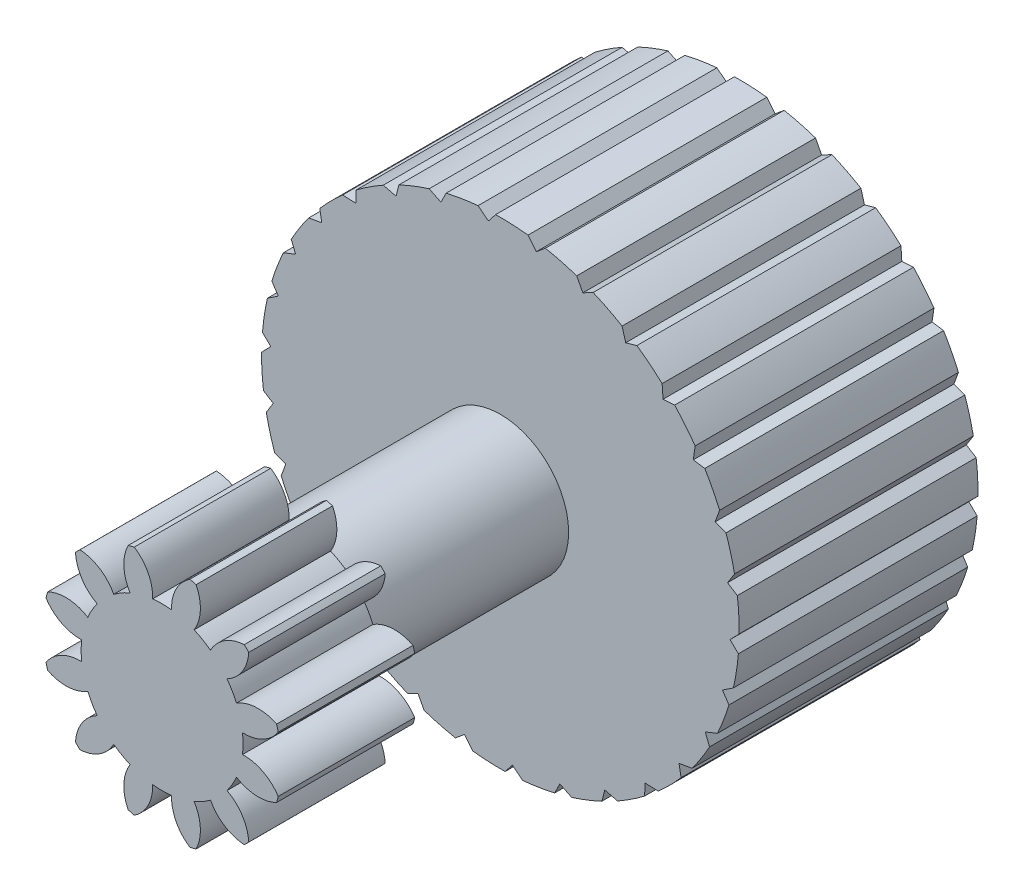
SolidWorks part; units mm, degrees
ref_plane "Front Plane" through (0, 0, 0) normal (0, 0, 1) x (1, 0, 0)
ref_plane "Top Plane" through (0, 0, 0) normal (0, 1, 0) x (1, 0, 0)
ref_plane "Right Plane" through (0, 0, 0) normal (1, 0, 0) x (0, 0, -1)
other "Configuration Table"
sketch "Sketch1" plane through (0, 0, 0) normal (0, 0, 1) x (1, 0, 0)
  circle A0 centre (0, 0) radius 1
  dimension "D1" = 2
extrude "Boss-Extrude1" add sketch "Sketch1" along normal blind 3
sketch "Sketch2" plane through (0, 0, 3) normal (0, 0, 1) x (1, 0, 0)
  arc A0 (-1.2279, 1.1338) -> (-0.9093, 0.6388) centre (-0.629, 1.1693) ccw
  arc A1 (-0.9093, 0.6388) -> (-1.0478, 0.3989) centre (0.0419, -0.0703) ccw
  arc A2 (-1.0478, 0.3989) -> (-1.6358, 0.4273) centre (-1.3671, -0.1091) ccw
  arc A3 (-1.6358, 0.4273) -> (-1.6599, 0.3375) centre (0.0419, -0.0703) ccw
  arc A4 (-1.6599, 0.3375) -> (-1.1365, 0.0682) centre (-1.1589, 0.6677) ccw
  arc A5 (-1.1365, 0.0682) -> (-1.1365, -0.2088) centre (0.0419, -0.0703) ccw
  arc A6 (-1.1365, -0.2088) -> (-1.6599, -0.4782) centre (-1.1589, -0.8084) ccw
  arc A7 (-1.6599, -0.4782) -> (-1.6358, -0.568) centre (0.0419, -0.0703) ccw
  arc A8 (-1.6358, -0.568) -> (-1.0478, -0.5396) centre (-1.3671, -0.0316) ccw
  arc A9 (-1.0478, -0.5396) -> (-0.9093, -0.7795) centre (0.0419, -0.0703) ccw
  arc A10 (-0.9093, -0.7795) -> (-1.2279, -1.2745) centre (-0.629, -1.31) ccw
  arc A11 (-1.2279, -1.2745) -> (-1.1622, -1.3402) centre (0.0419, -0.0703) ccw
  arc A12 (-1.1622, -1.3402) -> (-0.6672, -1.0216) centre (-1.1977, -0.7413) ccw
  arc A13 (-0.6672, -1.0216) -> (-0.4273, -1.1601) centre (0.0419, -0.0703) ccw
  arc A14 (-0.4273, -1.1601) -> (-0.4557, -1.7481) centre (0.0807, -1.4794) ccw
  arc A15 (-0.4557, -1.7481) -> (-0.3659, -1.7722) centre (0.0419, -0.0703) ccw
  arc A16 (-0.3659, -1.7722) -> (-0.0966, -1.2487) centre (-0.6961, -1.2712) ccw
  arc A17 (-0.0966, -1.2487) -> (0.1804, -1.2487) centre (0.0419, -0.0703) ccw
  arc A18 (0.1804, -1.2487) -> (0.4498, -1.7722) centre (0.78, -1.2712) ccw
  arc A19 (0.4498, -1.7722) -> (0.5396, -1.7481) centre (0.0419, -0.0703) ccw
  arc A20 (0.5396, -1.7481) -> (0.5112, -1.1601) centre (0.0032, -1.4794) ccw
  arc A21 (0.5112, -1.1601) -> (0.7511, -1.0216) centre (0.0419, -0.0703) ccw
  arc A22 (0.7511, -1.0216) -> (1.2461, -1.3402) centre (1.2816, -0.7413) ccw
  arc A23 (1.2461, -1.3402) -> (1.3118, -1.2745) centre (0.0419, -0.0703) ccw
  arc A24 (1.3118, -1.2745) -> (0.9932, -0.7795) centre (0.7129, -1.31) ccw
  arc A25 (0.9932, -0.7795) -> (1.1317, -0.5396) centre (0.0419, -0.0703) ccw
  arc A26 (1.1317, -0.5396) -> (1.7197, -0.568) centre (1.4509, -0.0316) ccw
  arc A27 (1.7197, -0.568) -> (1.7437, -0.4782) centre (0.0419, -0.0703) ccw
  arc A28 (1.7437, -0.4782) -> (1.2203, -0.2088) centre (1.2428, -0.8084) ccw
  arc A29 (1.2203, -0.2088) -> (1.2203, 0.0682) centre (0.0419, -0.0703) ccw
  arc A30 (1.2203, 0.0682) -> (1.7437, 0.3375) centre (1.2428, 0.6677) ccw
  arc A31 (1.7437, 0.3375) -> (1.7197, 0.4273) centre (0.0419, -0.0703) ccw
  arc A32 (1.7197, 0.4273) -> (1.1317, 0.3989) centre (1.4509, -0.1091) ccw
  arc A33 (1.1317, 0.3989) -> (0.9932, 0.6388) centre (0.0419, -0.0703) ccw
  arc A34 (0.9932, 0.6388) -> (1.3118, 1.1338) centre (0.7129, 1.1693) ccw
  arc A35 (1.3118, 1.1338) -> (1.2461, 1.1995) centre (0.0419, -0.0703) ccw
  arc A36 (1.2461, 1.1995) -> (0.7511, 0.8809) centre (1.2816, 0.6006) ccw
  arc A37 (0.7511, 0.8809) -> (0.5112, 1.0194) centre (0.0419, -0.0703) ccw
  arc A38 (0.5112, 1.0194) -> (0.5396, 1.6074) centre (0.0032, 1.3387) ccw
  arc A39 (0.5396, 1.6074) -> (0.4498, 1.6315) centre (0.0419, -0.0703) ccw
  arc A40 (0.4498, 1.6315) -> (0.1804, 1.108) centre (0.78, 1.1305) ccw
  arc A41 (0.1804, 1.108) -> (-0.0966, 1.108) centre (0.0419, -0.0703) ccw
  arc A42 (-0.0966, 1.108) -> (-0.3659, 1.6315) centre (-0.6961, 1.1305) ccw
  arc A43 (-0.3659, 1.6315) -> (-0.4557, 1.6074) centre (0.0419, -0.0703) ccw
  arc A44 (-0.4557, 1.6074) -> (-0.4273, 1.0194) centre (0.0807, 1.3387) ccw
  arc A45 (-0.4273, 1.0194) -> (-0.6672, 0.8809) centre (0.0419, -0.0703) ccw
  arc A46 (-0.6672, 0.8809) -> (-1.1622, 1.1995) centre (-1.1977, 0.6006) ccw
  arc A47 (-1.1622, 1.1995) -> (-1.2279, 1.1338) centre (0.0419, -0.0703) ccw
extrude "Boss-Extrude2" add sketch "Sketch2" along normal blind 2
sketch "Sketch3" plane through (0, 0, 0) normal (0, 0, -1) x (-1, 0, 0)
  circle A0 centre (0, 0) radius 3.5
  dimension "D1" = 7
extrude "Boss-Extrude3" add sketch "Sketch3" along normal blind 3.5
sketch "Sketch4" plane through (0, 0, -3.5) normal (0, 0, -1) x (-1, 0, 0)
  line L0 (0.0701, 3.4993) -> (0.1754, 3.3654)
  line L1 (0.1754, 3.3654) -> (0.3272, 3.4847)
  line L2 (0.3272, 3.4847) -> (0.3272, 3.8161)
  line L3 (0.3272, 3.8161) -> (0.0701, 3.8161)
  line L4 (0.0701, 3.8161) -> (0.0701, 3.4993)
  circle A0 centre (0, 0) radius 3.5 construction
extrude "Cut-Extrude1" cut sketch "Sketch4" against normal blind 5
pattern_circular "CirPattern1" count 30 over 360 about axis through (0, 0, 0) along (0, 0, 1) of "Cut-Extrude1"
scale "Scale 1" scale about origin uniform scaling yes scale factor 0.7
